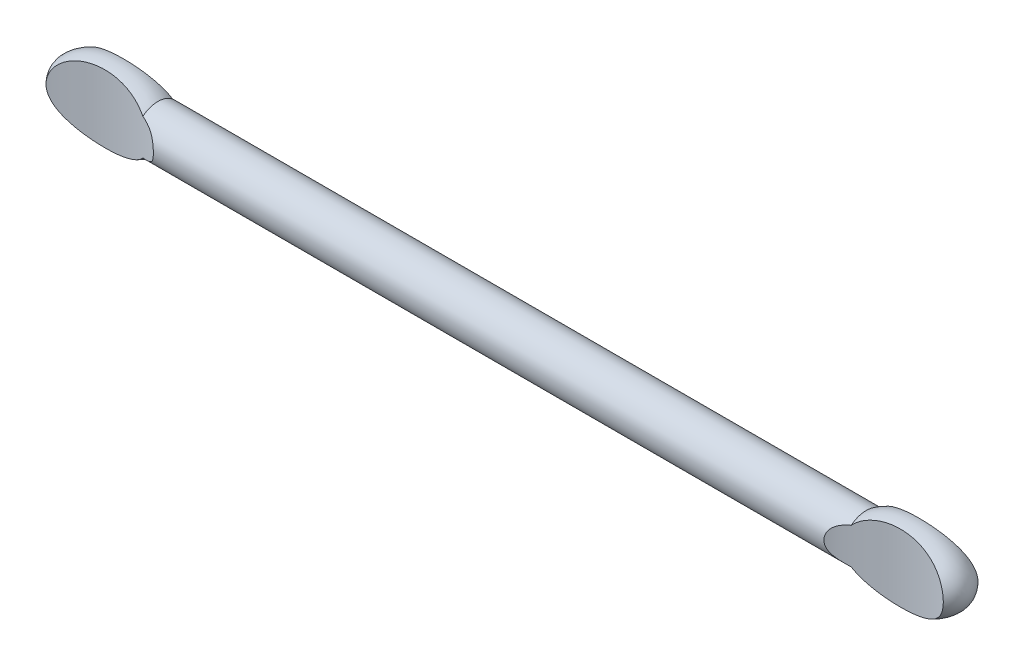
from build123d import *

# Parameters (mm, degrees)
SKETCH1_R           = 5
BOSS_EXTRUDE1_DEPTH = 85
SKETCH4_RX          = 15
SKETCH4_RY          = 5.5
CUT_EXTRUDE1_DEPTH  = 85


with BuildPart() as part:
    # Sketch1 → Boss-Extrude1 (new, symmetric)
    with BuildSketch(Plane(origin=(0, 0, 0), x_dir=(0, 0, -1), z_dir=(1, 0, 0))):
        Circle(SKETCH1_R)
    extrude(amount=BOSS_EXTRUDE1_DEPTH, both=True)

    # Sketch3 → Revolve3 (revolve)
    with BuildSketch(Plane(origin=(0, 0, 0), x_dir=(1, 0, 0), z_dir=(0, 1, 0))):
        with BuildLine():
            Line((97.5, 0), (72.5, 0))
            add(Edge.make_bspline(
                [(97.5, 0), (97.5, 7.5), (85, 7.5), (72.5, 7.5), (72.5, 0)],
                knots=[0, 0, 0, 1.570796327, 1.570796327, 3.141592654, 3.141592654, 3.141592654], degree=2, weights=[1, 0.707106781, 1, 0.707106781, 1]))
        make_face()
    revolve3 = revolve(axis=Axis((85, 0, 0), (1, 0, 0)))

    # Sketch4 → Cut-Extrude1 (cut, symmetric)
    with BuildSketch(Plane(origin=(0, 0, 0), x_dir=(1, 0, 0), z_dir=(0, 1, 0))):
        with Locations((85, 7.5)):
            Ellipse(SKETCH4_RX, SKETCH4_RY)
        with Locations((85, -7.5)):
            Ellipse(SKETCH4_RX, SKETCH4_RY)
    cut_extrude1 = extrude(amount=CUT_EXTRUDE1_DEPTH, both=True, mode=Mode.SUBTRACT)

    # Mirror1: Revolve3, Cut-Extrude1 across plane
    add(revolve3.mirror(Plane(origin=(0, 0, 0), x_dir=(0, 0, 1), z_dir=(1, 0, 0))))
    add(cut_extrude1.mirror(Plane(origin=(0, 0, 0), x_dir=(0, 0, 1), z_dir=(1, 0, 0))), mode=Mode.SUBTRACT)


solid = part.part
